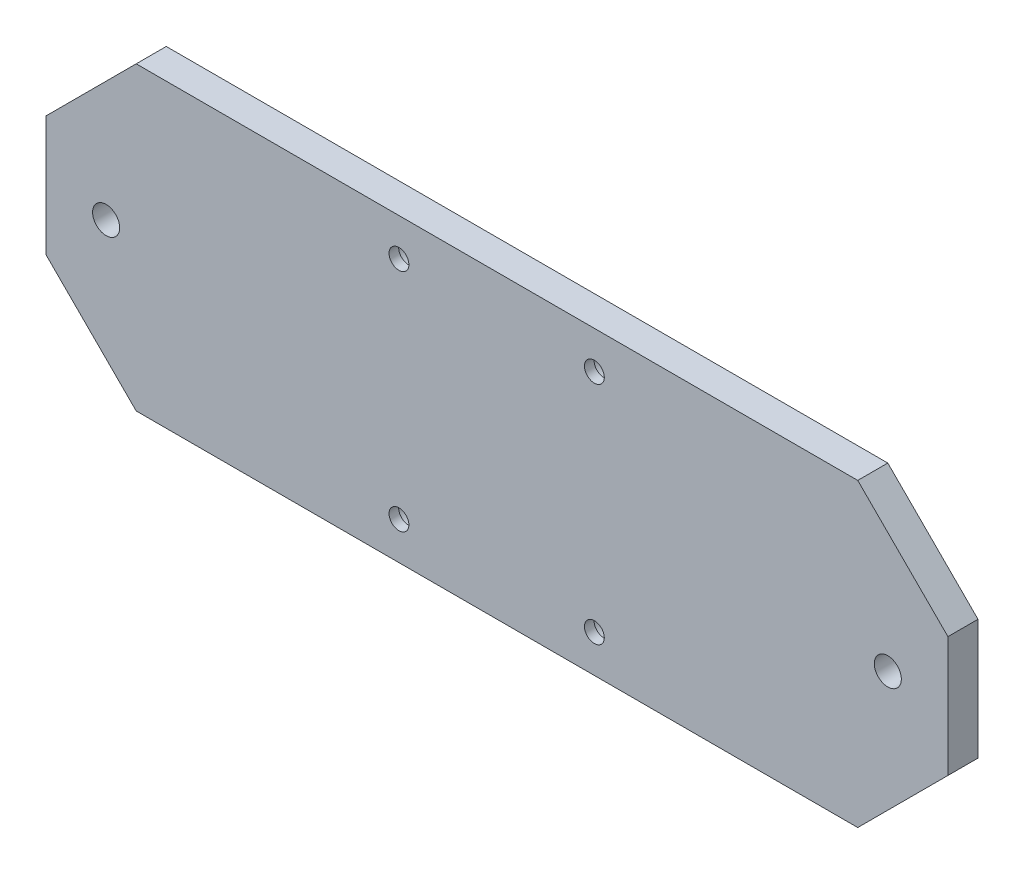
SolidWorks part; units mm, degrees
ref_plane "前视基准面" through (0, 0, 0) normal (0, 0, 1) x (1, 0, 0)
ref_plane "上视基准面" through (0, 0, 0) normal (0, 1, 0) x (1, 0, 0)
ref_plane "右视基准面" through (0, 0, 0) normal (1, 0, 0) x (0, 0, -1)
sketch "草图1" plane through (0, 0, 0) normal (0, 0, 1) x (1, 0, 0)
  line L1 (150, -50) -> (-150, -50)
  line L2 (150, -50) -> (150, 50)
  line L3 (150, 50) -> (-150, 50)
  line L4 (-150, -50) -> (-150, 50)
  line L5 (150, -50) -> (-150, 50) construction
  line L6 (150, 50) -> (-150, -50) construction
  point P0 (0, 0)
  dimension "D1" = 100
  dimension "D2" = 300
extrude "凸台-拉伸1" add sketch "草图1" along normal blind 10
hole_wizard "打孔尺寸(%根据)内六角圆柱头螺钉的类型1" positions "草图2" profile "草图3" counterbore size "M6" standard "GB" end condition up to next
sketch "草图2" plane through (0, 0, 0) normal (0, 0, -1) x (-1, 0, 0)
  point P0 (32.6, -37.5)
  point P3 (-32.4, -37.5)
  point P6 (-32.4, 37.5)
  point P9 (32.6, 37.5)
sketch "草图3" plane through (-32.6, -37.5, 0) normal (1, 0, 0) x (0, 1, 0)
  line L0 (0, 0) -> (0, 10)
  line L1 (0, 10) -> (3.3, 10)
  line L3 (3.3, 10) -> (3.3, 6.8)
  line L4 (3.3, 6.8) -> (5.5, 6.8)
  line L5 (5.5, 6.8) -> (5.5, 0)
  line L7 (5.5, 0) -> (0, 0)
  line L11 (0, -6.35) -> (0, 107.95) construction
  dimension "通孔孔直径" = 6.6
  dimension "通孔孔深度" = 10
  dimension "柱形沉头孔直径" = 11
  dimension "柱形沉头孔深度" = 6.8
hole_wizard "M8 间隙孔1" positions "草图4" profile "草图6" hole size "M8" standard "GB" end condition up to next
sketch "草图4" plane through (0, 0, 0) normal (0, 0, -1) x (-1, 0, 0)
  line L0 (-130, 0) -> (0, 0) construction
  line L1 (0, 0) -> (130, 0) construction
  point P3 (-130, 0)
  point P6 (130, 0)
  dimension "D1" = 130
sketch "草图6" plane through (130, 0, 0) normal (1, 0, 0) x (0, 1, 0)
  line L0 (0, 0) -> (0, 10)
  line L1 (0, 10) -> (4.5, 10)
  line L2 (4.5, 10) -> (4.5, 0)
  line L5 (4.5, 0) -> (0, 0)
  line L11 (0, -6.35) -> (0, 107.95) construction
  dimension "通孔孔直径" = 9
  dimension "通孔孔深度" = 10
chamfer "倒角1" distance 30 angle 45 4 edges at (150, -50, 5) (150, 50, 5) (-150, 50, 5) (-150, -50, 5)
